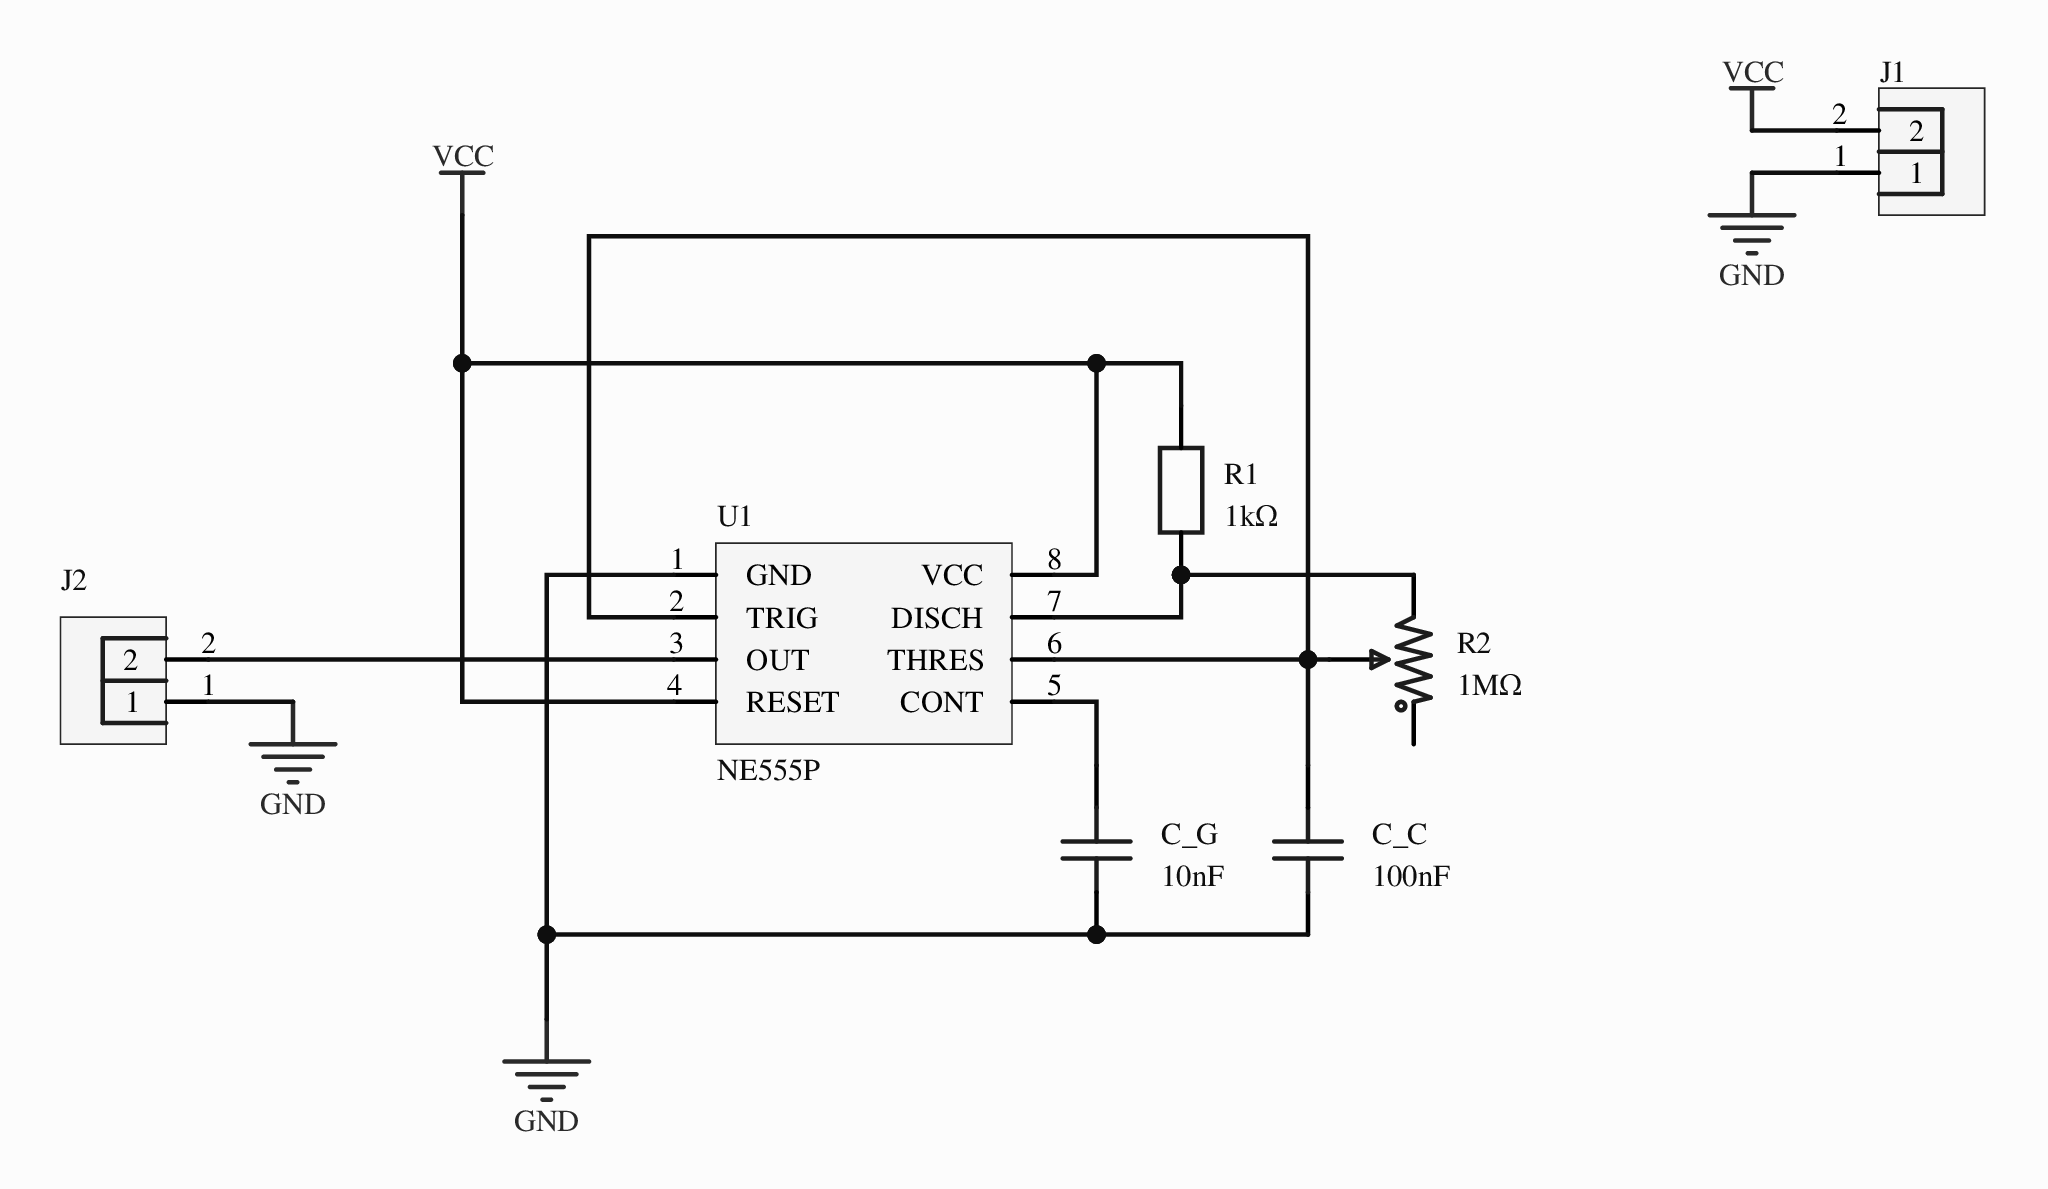
[diagram p0: MISC51049-3.schdoc]
# Altium project MISC51049-2.PrjPcb
1 sheet, 7 parts. Net scope: global (net labels, ports and power ports of the same name join across sheets).
Board file: MISC51049.pcbdoc

## Sheet MISC51049-3.schdoc
size 210 x 148 mm; Version: V1.0; @Project Name: MISC51049; @Update Date: 2026-10-07; @Create Date: 2026-10-07; @Board Name: MISC51049; @Create Time: 12:44:54; @Page Count: 1; @Page No: 1; @Schematic Name: MISC51049; @Update Time: 12:44:54; Size: A4

### Parts
C_C  100nF  [CAP-TH_L5.0-W2.5-P5.00-D1.0]
C_G  10nF  [CAP-TH_L5.5-W3.0-P5.00-D0.6]
J1  (no value)  [HDR-TH_2P-P2.54-V-M-1]
J2  (no value)  [HDR-TH_2P-P2.54-V-M-1]
R1  1kΩ  [RES-TH_BD2.7-L6.2-P10.20-D0.4]
R2  1MΩ  [RES-ADJ-TH_RM063-103]
U1  NE555P  [DIP-8_L9.8-W6.6-P2.54-LS7.6-BL]

### Nets
GND: C_C.1 C_G.1 J1.1 J2.1 U1.1(GND)
VCC: J1.2 R1.2 U1.4(RESET) U1.8(VCC)
NetC_C_2: C_C.2 R2.2 U1.2(TRIG) U1.6(THRES)
NetC_G_2: C_G.2 U1.5(CONT)
NetJ2_2: J2.2 U1.3(OUT)
NetR1_1: R1.1 R2.3 U1.7(DISCH)

Not connected (* = marked no-connect by the designer): R2 1*

### Library data of the parts
C_C = CC1H104MC1FD3F6C10MF: Capacitance: 100nF; tolerance: ±20%; rated voltage: 50V; temperature coefficient: Y5V;; Manufacturer: Dersonic(德尔创); 3D Model: 08e3d7481fc7486bb1b263873f51e1e10819f05c4eef4c71ace90d822a990e87; 3D Model Transform: 224.652,98.425,0,0,0,0,-0.005,0,-137.795; Pin Spacing: 5.08mm; Body Thickness: 2.2mm; AddInBom: yes; ModelName: CAP-TH_BD5.0-W2.5-P5.08; Symbol: CC1H104MC1FD3F6C10MF; Device: CC1H104MC1FD3F6C10MF; LCSC Part Name: 100nF ±20% 50V; Supplier Part: C254085; Manufacturer Part: CC1H104MC1FD3F6C10MF; Supplier Footprint: 插件,P=5.08mm; JLCPCB Part Class: Extended Part; Datasheet: https://item.szlcsc.com/datasheet/CC1H104MC1FD3F6C10MF/248635.html; Supplier: LCSC; Value: 100nF; Tolerance: ±20%; Voltage Rating: 50V; Temperature Coefficient: Y5V; Diameter: 6mm; FootprintName: CAP-TH_L5.0-W2.5-P5.00-D1.0; ConvertToPcb: yes
C_G = DCT103M22Y5UF6FJ5A0: Capacitance: 10nF; tolerance: ±20%; rated voltage: 50V; temperature coefficient: Y5U;; Manufacturer: SHM(南方宏明); 3D Model: 8f31db7ace7a416e97923e9ed245e9d50819f05c4eef4c71ace90d822a990e87; 3D Model Transform: 232.661,127.248,0,0,0,0,-0.005,0,-196.85; Pin Spacing: 5mm; AddInBom: yes; Symbol: DCT103M22Y5UF6FJ5A0; Device: DCT103M22Y5UF6FJ5A0; LCSC Part Name: 10nF ±20% 50V; Supplier Part: C2896035; Manufacturer Part: DCT103M22Y5UF6FJ5A0; Supplier Footprint: 插件,P=5mm; JLCPCB Part Class: Extended Part; Datasheet: https://item.szlcsc.com/datasheet/DCT103M22Y5UF6FJ5A0/3138584.html; Supplier: LCSC; Value: 10nF; Tolerance: ±20%; Voltage Rating: 50V; Temperature Coefficient: Y5U; FootprintName: CAP-TH_L5.5-W3.0-P5.00-D0.6; ConvertToPcb: yes; ModelName: CAP-TH_L5.5-W3.0-P5.00-D0.6
J1 J2 = HDR-M_2.54_1x2P: Symbol: 210S-1*2P L=11.6MMGold-plated black; 3D Model: 79b2e9f2d70a4d68a1b7098f27c6d4c50819f05c4eef4c71ace90d822a990e87; 3D Model Transform: 200,100,0,0,0,0,0,0,-118.11; ConvertToPcb: yes; ModelName: HDR-M-2.54_1x2; Device: HDR-M_2.54_1x2P; Supplier Part: C124375; Supplier Footprint: 插件; FootprintName: HDR-TH_2P-P2.54-V-M-1; AddInBom: yes
R1 = MF1/4W-1K±1%-ST52: Resistor type: metal film resistor; resistance: 1kΩ; tolerance: ±1%; power: 250mW; temperature coefficient: ±100ppm/℃;; Manufacturer: VO(翔胜); 3D Model: f91fbe0e2e6f409498f09f811e4616fe0819f05c4eef4c71ace90d822a990e87; 3D Model Transform: 417.322,106.221,0,0,0,0,0,0,-196.85; Voltage-Supply(Max): 250V; AddInBom: yes; Symbol: MF1/4W-1K±1%-ST52; Device: MF1/4W-1K±1%-ST52; LCSC Part Name: 金属膜电阻 1kΩ ±1% 250mW; Supplier Part: C2903245; Manufacturer Part: MF1/4W-1K±1%-ST52; Supplier Footprint: 插件,D2.7xL6.2mm; JLCPCB Part Class: Extended Part; Datasheet: https://item.szlcsc.com/datasheet/MF1%252F4W-1K%25C2%25B11%2525-ST52/3158996.html; Supplier: LCSC; Type: Metal film resistor; Value: 1kΩ; Tolerance: ±1%; Power(Watts): 250mW; Temperature Coefficient: ±100ppm/℃; Operating Temperature: -55℃~+155℃; FootprintName: RES-TH_BD2.7-L6.2-P10.20-D0.4; ConvertToPcb: yes; ModelName: RES-TH_BD2.7-L6.2-P10.20-D0.4
R2 = RM063-105(1M): Resistance: 1MΩ; tolerance: ±25%; power: 100mW;; Manufacturer: BOCHEN(博晨); 3D Model: c2e79538aa8f4a14bd3d91be27bc95d30819f05c4eef4c71ace90d822a990e87; 3D Model Transform: 255.905,230.194,0,0,0,0,0,-52.48,-137.795; Voltage Rating: 50V; AddInBom: yes; Symbol: RM063-105(1M); Device: RM063-105(1M); LCSC Part Name: 1MΩ ±25%; Supplier Part: C5205038; Manufacturer Part: RM063-105(1M); Supplier Footprint: 插件,6.4x5.2mm; JLCPCB Part Class: Extended Part; Datasheet: https://item.szlcsc.com/datasheet/RM063-105(1M)/5896396.html; Supplier: LCSC; Value: 1MΩ; Tolerance: ±25%; Power(Watts): 100mW; FootprintName: RES-ADJ-TH_RM063-103; ConvertToPcb: yes; ModelName: RES-ADJ-TH_RM063-103
U1 = NE555P: Precision timing circuits that generate accurate time delays or oscillations. In delay or monostable mode, the timing interval is set by a single external resistor and capacitor network. In astable mode, frequency and duty cycle are set by two external resistors and one external capacitor.; Manufacturer: TI(德州仪器); 3D Model: db2af726fcec488f8bf8e467aca974b30819f05c4eef4c71ace90d822a990e87; 3D Model Transform: 385.826,311.8104,0,0,0,0,-1.693,0,-137.795; AddInBom: yes; ModelName: DIP-8_L9.8-W6.6-H3.5-LS7.62-P2.54; Symbol: NE555P; Device: NE555P; LCSC Part Name: NE555P; Supplier Part: C46749; Manufacturer Part: NE555P; Supplier Footprint: DIP-8; JLCPCB Part Class: Extended Part; Supplier: LCSC; FootprintName: DIP-8_L9.8-W6.6-P2.54-LS7.6-BL; ConvertToPcb: yes